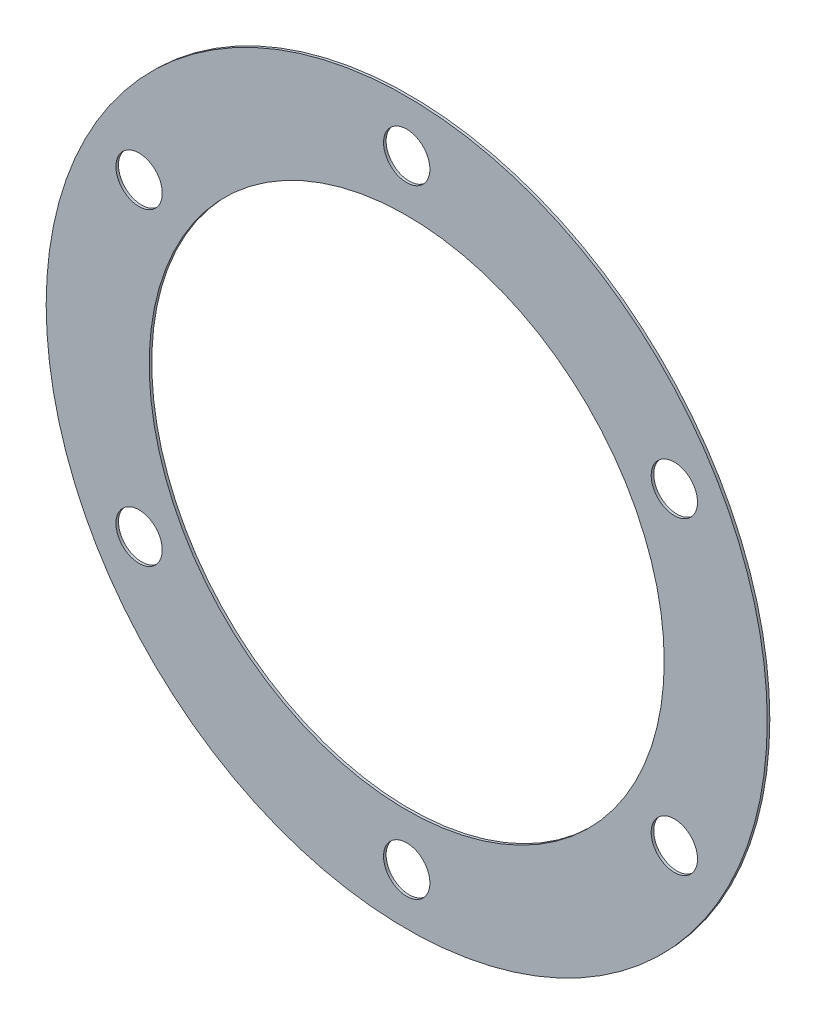
SolidWorks part; units mm, degrees
ref_plane "Front Plane" through (0, 0, 0) normal (0, 0, 1) x (1, 0, 0)
ref_plane "Top Plane" through (0, 0, 0) normal (0, 1, 0) x (1, 0, 0)
ref_plane "Right Plane" through (0, 0, 0) normal (1, 0, 0) x (0, 0, -1)
sketch "Sketch1" plane through (0, 0, 0) normal (0, 0, 1) x (1, 0, 0)
  circle A0 centre (0, 0) radius 50
  circle A1 centre (0, 0) radius 70
  dimension "D1" = 100
  dimension "D2" = 140
extrude "Boss-Extrude1" add sketch "Sketch1" along normal blind 0.5
sketch "Sketch2" plane through (0, 0, 0.5) normal (0, 0, 1) x (1, 0, 0)
  circle A0 centre (0, 60) radius 4.5
  dimension "D2" = 9
  dimension "D1" = 60
extrude "Cut-Extrude1" cut sketch "Sketch2" against normal through all
pattern_circular "CirPattern1" count 6 over 360 about axis through (0, 0, 0) along (0, 0, 1) of "Cut-Extrude1"
